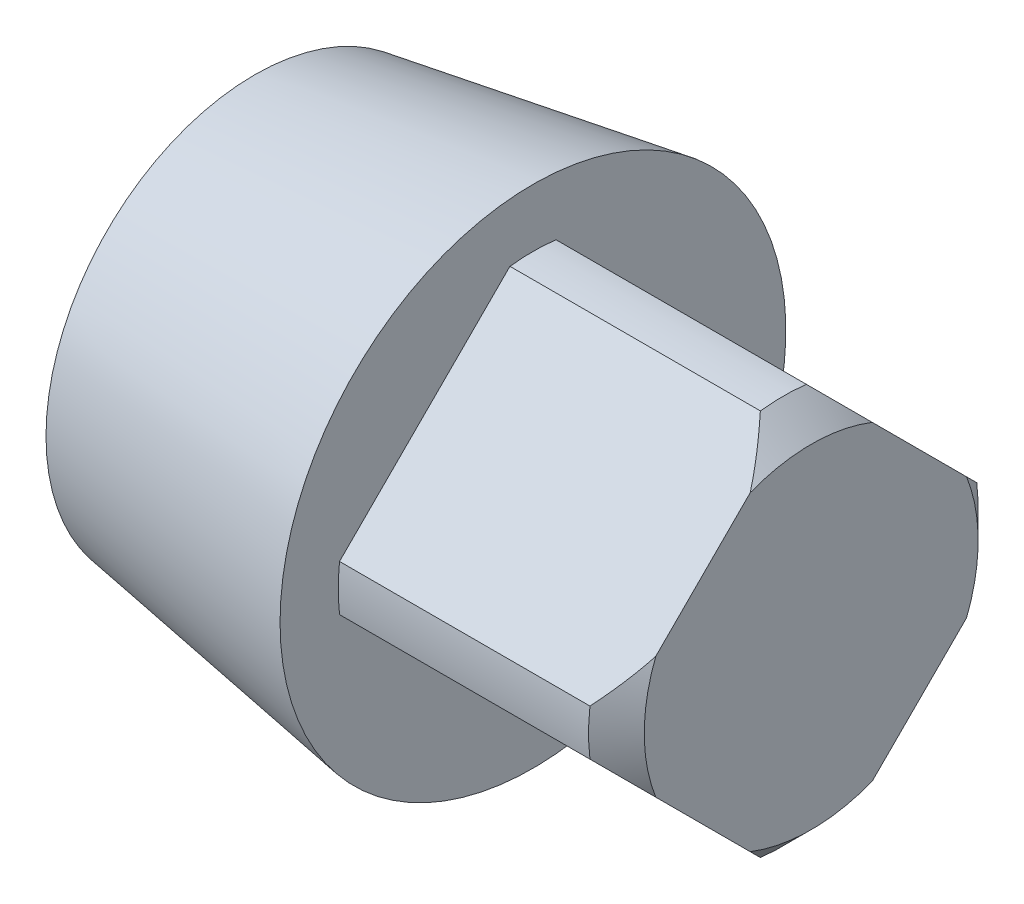
from build123d import *

# Parameters (mm, degrees)
CHAMFER1_SIZE      = 2
CUT_EXTRUDE1_START = -20
CUT_EXTRUDE1_DEPTH = 20
CIRPATTERN1_COUNT  = 4


with BuildPart() as part:
    # Sketch1 → Revolve1 (revolve)
    with BuildSketch(Plane.XY, mode=Mode.PRIVATE) as revolve1_sk:
        Polygon((0, 0), (20, 0), (40, 0), (40, 14), (20, 14), (20, 18.177165354), (0, 15), align=None)
    revolve(revolve1_sk.sketch.rotate(Axis((20, 0, 0), (1, 0, 0)), 90), axis=Axis((20, 0, 0), (1, 0, 0)))

    # Chamfer1
    chamfer1_edges = [part.edges().sort_by_distance(p)[0] for p in [
        (40, 0, -14),
    ]]
    chamfer(chamfer1_edges, length=CHAMFER1_SIZE)

    # Sketch2 → Cut-Extrude1 (cut)
    with BuildSketch(Plane(origin=(40, 0, 0), x_dir=(0, 0, -1), z_dir=(1, 0, 0)).offset(CUT_EXTRUDE1_START)):
        with BuildLine():
            Line((11.169339585, 4.387009601), (13.90189895, 1.654450236))
            ThreePointArc((13.90189895, 1.654450236), (9.899494937, 9.899494937), (1.654450236, 13.90189895))
            Line((1.654450236, 13.90189895), (4.387009601, 11.169339585))
            ThreePointArc((4.387009601, 11.169339585), (8.485281374, 8.485281374), (11.169339585, 4.387009601))
        make_face()
        with BuildLine():
            Line((4.387009601, 11.169339585), (11.169339585, 4.387009601))
            ThreePointArc((11.169339585, 4.387009601), (8.485281374, 8.485281374), (4.387009601, 11.169339585))
        make_face()
    cut_extrude1 = extrude(amount=CUT_EXTRUDE1_DEPTH, mode=Mode.SUBTRACT)

    # CirPattern1: Cut-Extrude1 ×4 about axis
    cirpattern1_axis = Axis((0, 0, 0), (1, 0, 0))
    for i in range(1, CIRPATTERN1_COUNT):
        add(cut_extrude1.rotate(cirpattern1_axis, i * 360 / CIRPATTERN1_COUNT), mode=Mode.SUBTRACT)


solid = part.part
